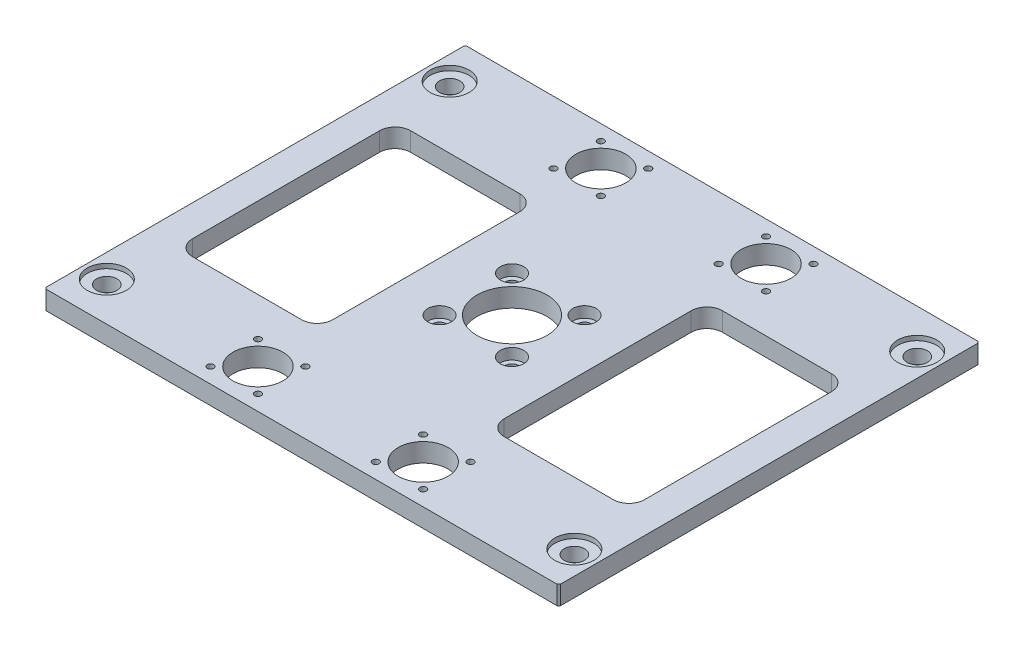
SolidWorks part; units mm, degrees
material "S45C"
ref_plane "Front Plane" through (0, 0, 0) normal (0, 0, 1) x (1, 0, 0)
ref_plane "Top Plane" through (0, 0, 0) normal (0, 1, 0) x (1, 0, 0)
ref_plane "Right Plane" through (0, 0, 0) normal (1, 0, 0) x (0, 0, -1)
sketch "Sketch1" plane through (0, 0, 0) normal (0, 1, 0) x (1, 0, 0)
  line L1 (-165, -135) -> (165, -135)
  line L2 (-165, -135) -> (-165, 135)
  line L3 (-165, 135) -> (165, 135)
  line L4 (165, -135) -> (165, 135)
  line L5 (-165, -135) -> (165, 135) construction
  line L6 (-165, 135) -> (165, -135) construction
  point P0 (0, 0)
  dimension "D1" = 330
  dimension "D2" = 270
extrude "Boss-Extrude1" add sketch "Sketch1" along normal mid plane 12
sketch "Sketch2" plane through (0, 6, 0) normal (0, 1, 0) x (1, 0, 0)
  line L0 (0, 0) -> (0, 139.4481) construction
  line L5 (0, 0) -> (-105.8517, 0) construction
  circle A0 centre (-53, 110) radius 16
  circle A1 centre (53, 110) radius 16
  circle A2 centre (53, -110) radius 16
  circle A3 centre (-53, -110) radius 16
  dimension "D1" = 32
  dimension "D2" = 106
  dimension "D3" = 220
extrude "Cut-Extrude1" cut sketch "Sketch2" against normal through all
sketch "Sketch3" plane through (0, 6, 0) normal (0, 1, 0) x (1, 0, 0)
  circle A0 centre (0, 0) radius 22.5
  dimension "D1" = 45
extrude "Cut-Extrude2" cut sketch "Sketch3" against normal through all
sketch "Sketch4" plane through (0, 6, 0) normal (0, 1, 0) x (1, 0, 0)
  line L0 (0, 0) -> (182.6517, 0) construction
  line L1 (0, 0) -> (0, 150.1483) construction
  line L2 (-165, 135) -> (-165, -135) construction
  line L3 (165, 135) -> (-165, 135) construction
  circle A0 centre (-150, 110) radius 12.5
  circle A1 centre (150, 110) radius 12.5
  circle A2 centre (150, -110) radius 12.5
  circle A3 centre (-150, -110) radius 12.5
  dimension "D1" = 25
  dimension "D2" = 15
  dimension "D3" = 25
extrude "Cut-Extrude3" cut sketch "Sketch4" against normal blind 3
hole_wizard "M12 Clearance Hole1" positions "Sketch5" profile "Sketch6" hole size "M12" standard "GB" end condition through all
sketch "Sketch5" plane through (0, -6, 0) normal (0, -1, 0) x (-1, 0, 0)
  point P0 (150, -110)
  point P3 (-150, -110)
  point P6 (150, 110)
  point P9 (-150, 110)
sketch "Sketch6" plane through (-150, -6, 110) normal (1, 0, 0) x (0, 0, -1)
  line L0 (0, 0) -> (0, 12)
  line L1 (0, 12) -> (6.5, 12)
  line L2 (6.5, 12) -> (6.5, 0)
  line L5 (6.5, 0) -> (0, 0)
  line L11 (0, -6.35) -> (0, 107.95) construction
  dimension "通孔孔直径" = 13
  dimension "通孔孔深度" = 12
hole_wizard "M5 Tapped Hole1" positions "Sketch7" profile "Sketch8" tap size "M5" standard "GB" end condition through all
sketch "Sketch7" plane through (0, 6, 0) normal (0, 1, 0) x (1, 0, 0)
  line L14 (-53, 110) -> (-196.07, 110) construction
  line L17 (-53, 110) -> (-53, 155.9259) construction
  line L18 (-53, 110) -> (-68.2028, 125.2028) construction
  line L21 (0, 0) -> (0, 177.0957) construction
  line L24 (0, 0) -> (-214.5584, 0) construction
  circle A0 centre (-53, 110) radius 21.5 construction
  point P264 (-68.2028, 125.2028)
  point P267 (-37.7972, 125.2028)
  point P268 (-37.7972, 94.7972)
  point P269 (-68.2028, 94.7972)
  point P293 (37.7972, 125.2028)
  point P294 (37.7972, 94.7972)
  point P295 (68.2028, 94.7972)
  point P296 (68.2028, 125.2028)
  point P298 (68.2028, -125.2028)
  point P299 (68.2028, -94.7972)
  point P300 (37.7972, -94.7972)
  point P301 (37.7972, -125.2028)
  point P302 (-37.7972, -125.2028)
  point P303 (-37.7972, -94.7972)
  point P304 (-68.2028, -94.7972)
  point P305 (-68.2028, -125.2028)
  dimension "D2" = 43
  dimension "D1" = 45
sketch "Sketch8" plane through (-68.2028, 6, 125.2028) normal (1, 0, 0) x (0, 0, 1)
  line L0 (0, 0) -> (0, 12)
  line L1 (0, 12) -> (2.1, 12)
  line L2 (2.1, 12) -> (2.1, 0)
  line L5 (2.1, 0) -> (0, 0)
  line L11 (0, -6.35) -> (0, 107.95) construction
  dimension "通孔螺纹孔钻头直径" = 4.2
  dimension "通孔螺纹孔钻头深度" = 12
cosmetic thread "Cosmetic thread 1" parameters "D2"=5
cosmetic thread "Cosmetic thread 2" parameters "D2"=5
cosmetic thread "Cosmetic thread 3" parameters "D2"=5
cosmetic thread "Cosmetic thread 4" parameters "D2"=5
cosmetic thread "Cosmetic thread 5" parameters "D2"=5
cosmetic thread "Cosmetic thread 6" parameters "D2"=5
cosmetic thread "Cosmetic thread 7" parameters "D2"=5
cosmetic thread "Cosmetic thread 8" parameters "D2"=5
cosmetic thread "Cosmetic thread 9" parameters "D2"=5
cosmetic thread "Cosmetic thread 10" parameters "D2"=5
cosmetic thread "Cosmetic thread 11" parameters "D2"=5
cosmetic thread "Cosmetic thread 12" parameters "D2"=5
cosmetic thread "Cosmetic thread 13" parameters "D2"=5
cosmetic thread "Cosmetic thread 14" parameters "D2"=5
cosmetic thread "Cosmetic thread 15" parameters "D2"=5
cosmetic thread "Cosmetic thread 16" parameters "D2"=5
hole_wizard "Hole size per socket head cap screw type 1" positions "Sketch9" profile "Sketch10" counterbore size "M8" standard "GB" end condition through all
sketch "Sketch9" plane through (0, 6, 0) normal (0, 1, 0) x (1, 0, 0)
  line L8 (-23.25, -23.25) -> (23.25, -23.25) construction
  line L9 (-23.25, -23.25) -> (-23.25, 23.25) construction
  line L10 (-23.25, 23.25) -> (23.25, 23.25) construction
  line L11 (23.25, -23.25) -> (23.25, 23.25) construction
  line L12 (-23.25, -23.25) -> (23.25, 23.25) construction
  line L13 (-23.25, 23.25) -> (23.25, -23.25) construction
  point P153 (0, 0)
  point P154 (23.25, 23.25)
  point P259 (-23.25, -23.25)
  point P260 (-23.25, 23.25)
  point P261 (23.25, -23.25)
  dimension "D1" = 46.5
sketch "Sketch10" plane through (0, 6, 0) normal (1, 0, 0) x (0, 0, 1)
  line L0 (0, 0) -> (0, 12)
  line L1 (0, 12) -> (4.5, 12)
  line L3 (4.5, 12) -> (4.5, 7)
  line L4 (4.5, 7) -> (7.5, 7)
  line L5 (7.5, 7) -> (7.5, 0)
  line L7 (7.5, 0) -> (0, 0)
  line L11 (0, -6.35) -> (0, 107.95) construction
  dimension "通孔孔直径" = 9
  dimension "通孔孔深度" = 12
  dimension "柱形沉头孔直径" = 15
  dimension "柱形沉头孔深度" = 7
chamfer "Chamfer1" distance 1 angle 45 4 edges at (-165, 0, 135) (-165, 0, -135) (165, 0, -135) (165, 0, 135)
sketch "Sketch11" plane through (0, 6, 0) normal (0, 1, 0) x (1, 0, 0)
  line L0 (0, 10) -> (0, 165.6809) construction
  line L1 (-10, 0) -> (-200.8881, 0) construction
  line L2 (-165, 134) -> (-165, -134) construction
  line L3 (-135, 70) -> (-65, 70)
  line L4 (-145, 60) -> (-145, -60)
  line L5 (-135, -70) -> (-65, -70)
  line L6 (-55, 60) -> (-55, -60)
  line L7 (55, 60) -> (55, -60)
  line L8 (135, -70) -> (65, -70)
  line L9 (145, 60) -> (145, -60)
  line L10 (135, 70) -> (65, 70)
  arc A0 (-145, -60) -> (-135, -70) centre (-135, -60) ccw
  arc A1 (-65, -70) -> (-55, -60) centre (-65, -60) ccw
  arc A2 (-55, 60) -> (-65, 70) centre (-65, 60) ccw
  arc A3 (-135, 70) -> (-145, 60) centre (-135, 60) ccw
  arc A4 (0, 10) -> (-10, 0) centre (-10, 10) cw construction
  arc A5 (0, 10) -> (10, 0) centre (10, 10) ccw construction
  arc A6 (135, 70) -> (145, 60) centre (135, 60) cw
  arc A7 (55, 60) -> (65, 70) centre (65, 60) cw
  arc A8 (65, -70) -> (55, -60) centre (65, -60) cw
  arc A9 (145, -60) -> (135, -70) centre (135, -60) cw
  point P12 (-145, -70)
  point P17 (-55, 70)
  point P20 (-145, 70)
  point P23 (0, 0)
  dimension "D4" = 10
  dimension "D5" = 10
  dimension "D1" = 90
  dimension "D2" = 20
  dimension "D3" = 140
extrude "Cut-Extrude4" cut sketch "Sketch11" against normal through all
